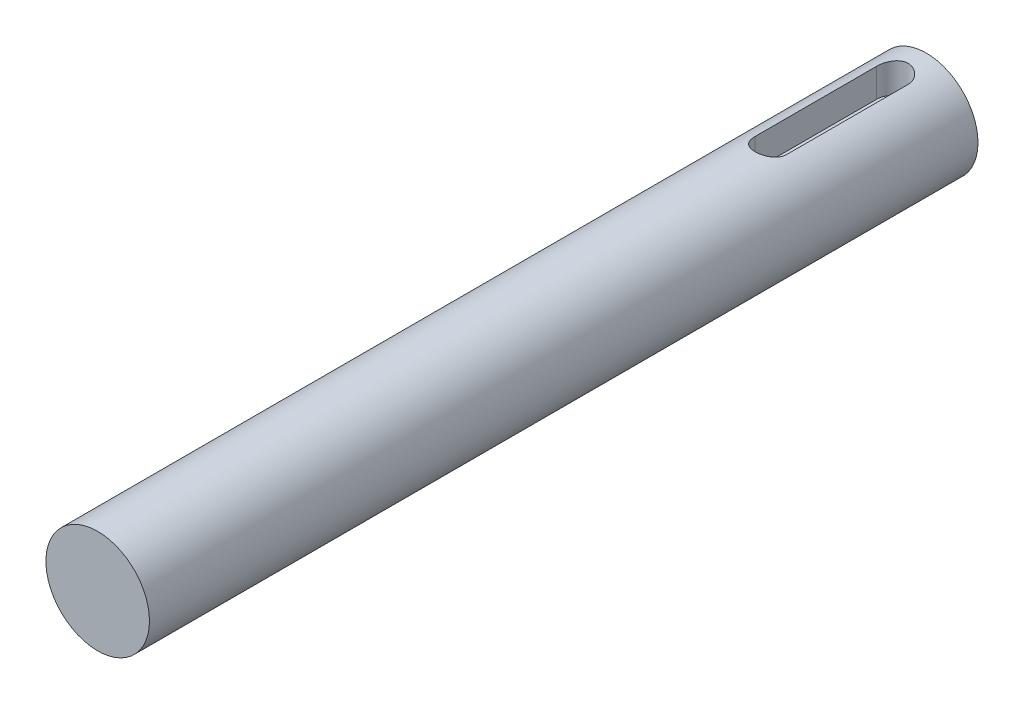
SolidWorks part; units mm, degrees
material "PBT general purpose"
ref_plane "Front Plane" through (0, 0, 0) normal (0, 0, 1) x (1, 0, 0)
ref_plane "Top Plane" through (0, 0, 0) normal (0, 1, 0) x (1, 0, 0)
ref_plane "Right Plane" through (0, 0, 0) normal (1, 0, 0) x (0, 0, -1)
sketch "Sketch1" plane through (0, 0, 0) normal (0, 0, 1) x (1, 0, 0)
  circle A0 centre (0, 0) radius 5
extrude "Boss-Extrude1" add sketch "Sketch1" along normal blind 80
ref_plane "Plane1" through (0, 5, 0) normal (0, 1, 0) x (1, 0, 0)
sketch "Sketch2" plane through (0, 5, 0) normal (0, 1, 0) x (1, 0, 0)
  line L2 (0, -15) -> (0, -3.2598) construction
  line L3 (-1.5196, -15) -> (-1.5196, -3.2598)
  line L4 (1.5196, -15) -> (1.5196, -3.2598)
  arc A0 (-1.5196, -15) -> (1.5196, -15) centre (0, -15) ccw
  arc A1 (1.5196, -3.2598) -> (-1.5196, -3.2598) centre (0, -3.2598) ccw
  point P5 (0, -9.1299)
extrude "Cut-Extrude2" cut sketch "Sketch2" against normal blind 3
